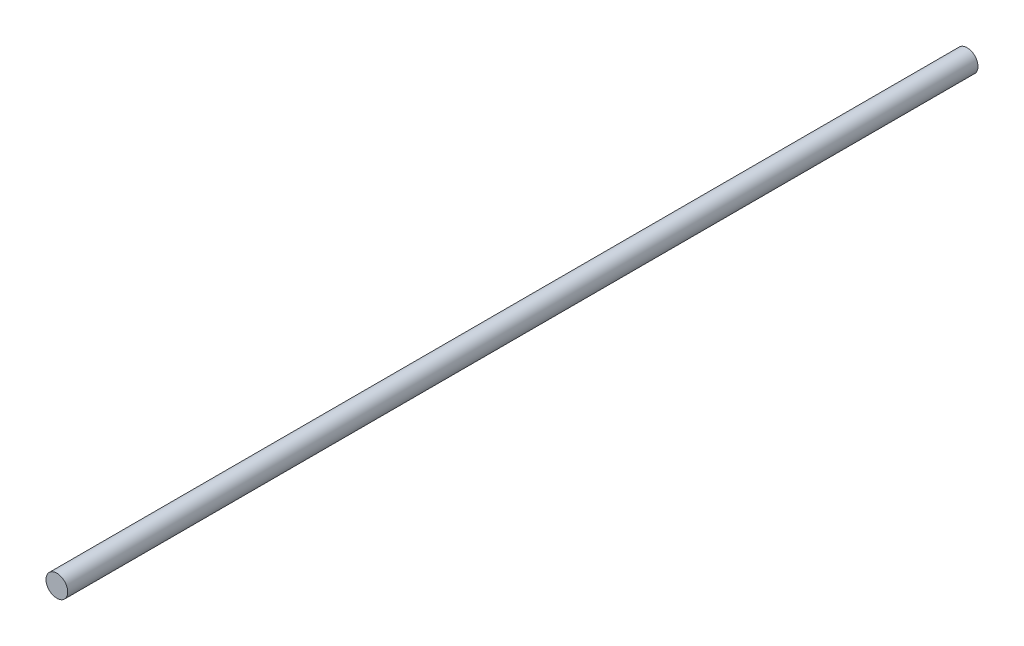
SolidWorks part; units mm, degrees
ref_plane "Front Plane" through (0, 0, 0) normal (0, 0, 1) x (1, 0, 0)
ref_plane "Top Plane" through (0, 0, 0) normal (0, 1, 0) x (1, 0, 0)
ref_plane "Right Plane" through (0, 0, 0) normal (1, 0, 0) x (0, 0, -1)
sketch "Sketch1" plane through (0, 0, 0) normal (0, 0, 1) x (1, 0, 0)
  circle A0 centre (0, 0) radius 8
  dimension "D1" = 16
extrude "Boss-Extrude1" add sketch "Sketch1" along normal blind 669
